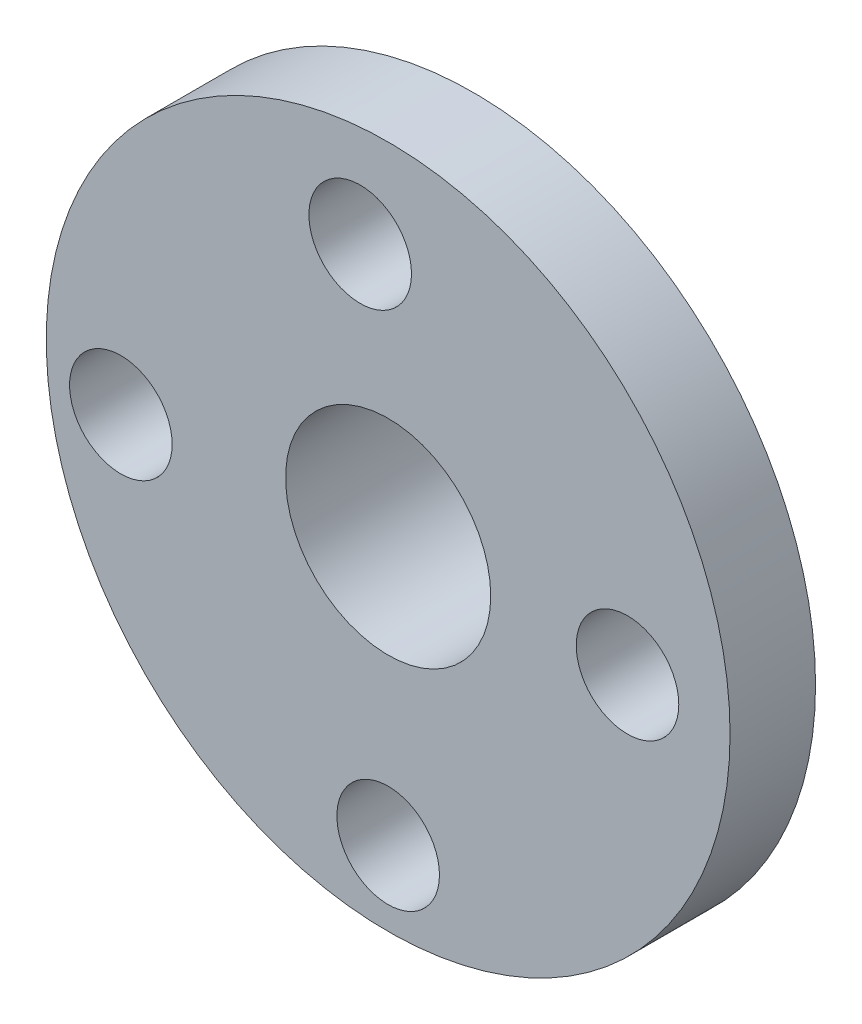
from build123d import *

# Parameters (mm, degrees)
SKETCH3_R                = 4.5
SKETCH3_R_2              = 3
BOSS_EXTRUDE1_DEPTH      = 3
BOSS_EXTRUDE2_DEPTH      = 2
BOSS_EXTRUDE2_DEPTH_BACK = 0.5
SKETCH4_R                = 10
SKETCH4_R_2              = 3
SKETCH5_R                = 1.5
CUT_EXTRUDE1_DEPTH       = 16


with BuildPart() as part:
    # Sketch3 → Boss-Extrude1 (new body)
    with BuildSketch(Plane.XY):
        Circle(SKETCH3_R)
        Circle(SKETCH3_R_2, mode=Mode.SUBTRACT)
    extrude(amount=BOSS_EXTRUDE1_DEPTH)

    # Sketch4 → Boss-Extrude2 (add, two sides: drawn at the far end of the back side and taken through both)
    with BuildSketch(Plane.XY.offset(3).offset(-BOSS_EXTRUDE2_DEPTH_BACK)):
        Circle(SKETCH4_R)
        Circle(SKETCH4_R_2, mode=Mode.SUBTRACT)
    extrude(amount=BOSS_EXTRUDE2_DEPTH + BOSS_EXTRUDE2_DEPTH_BACK)

    # Sketch5 → Cut-Extrude1 (cut, through all)
    with BuildSketch(Plane.XY.offset(5)):
        with Locations((7, 0)):
            Circle(SKETCH5_R)
        with Locations((-0.818126129, 7)):
            Circle(SKETCH5_R)
        with Locations((0, -7.818126129)):
            Circle(SKETCH5_R)
        with Locations((-7.818126129, -0.818126129)):
            Circle(SKETCH5_R)
    extrude(amount=-CUT_EXTRUDE1_DEPTH, mode=Mode.SUBTRACT)


solid = part.part
